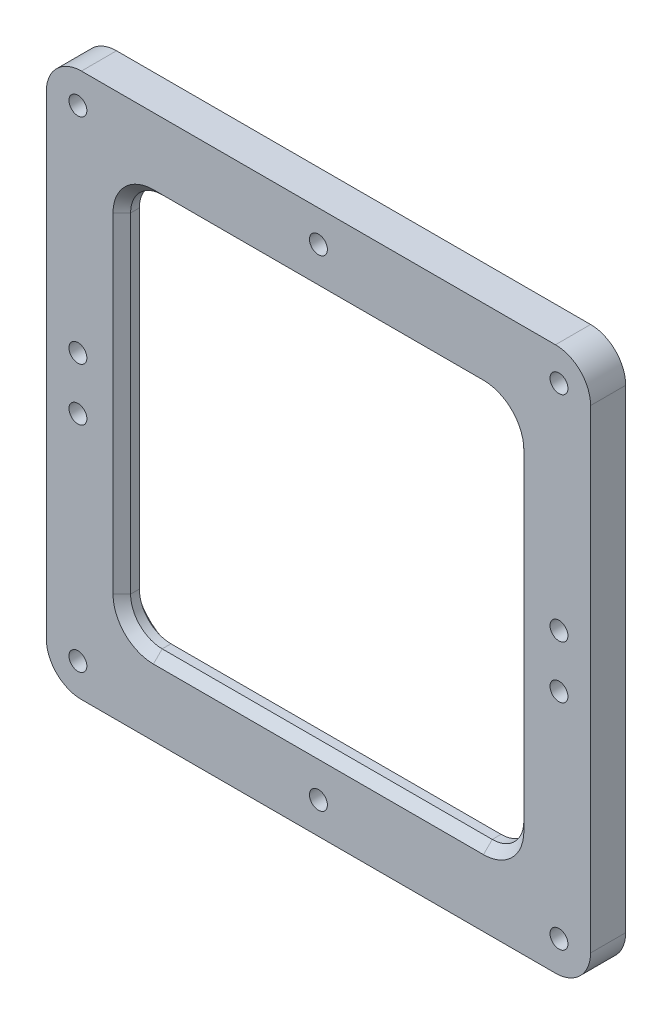
from build123d import *

# Parameters (mm, degrees)
SKETCH_1_W              = 310
SKETCH_1_H              = 310
EXTRUDE_1_DEPTH         = 20
FILLET_1_R              = 20
CUT_EXTRUDE_1_DEPTH     = 10
HOLE_WIZARD_M12_1_D     = 10.2
HOLE_WIZARD_M12_1_DEPTH = 15
HOLE_WIZARD_M12_1_TIP   = 3.064389157
CHAMFER_1_SIZE          = 5


with BuildPart() as part:
    # 草图1 → 凸台-拉伸1 (new body)
    with BuildSketch(Plane.XY):
        Rectangle(SKETCH_1_W, SKETCH_1_H)
        with BuildLine():
            Line((-94, 112), (94, 112))
            ThreePointArc((94, 112), (106.727922061, 106.727922061), (112, 94))
            Line((112, 94), (112, -94))
            ThreePointArc((112, -94), (106.727922061, -106.727922061), (94, -112))
            Line((94, -112), (-94, -112))
            ThreePointArc((-94, -112), (-106.727922061, -106.727922061), (-112, -94))
            Line((-112, -94), (-112, 94))
            ThreePointArc((-112, 94), (-106.727922061, 106.727922061), (-94, 112))
        make_face(mode=Mode.SUBTRACT)
    extrude(amount=EXTRUDE_1_DEPTH)

    # 圆角1
    fillet_1_edges = [part.edges().sort_by_distance(p)[0] for p in [
        (155, -155, 10),
        (-155, -155, 10),
        (-155, 155, 10),
        (155, 155, 10),
    ]]
    fillet(fillet_1_edges, radius=FILLET_1_R)

    # 草图2 → 切除-拉伸1 (cut)
    with BuildSketch(Plane(origin=(0, 0, 0), x_dir=(-1, 0, 0), z_dir=(0, 0, -1))):
        with BuildLine():
            Line((125.1, -95.1), (125.1, 95.1))
            ThreePointArc((125.1, 95.1), (116.313203436, 116.313203436), (95.1, 125.1))
            Line((95.1, 125.1), (-95.1, 125.1))
            ThreePointArc((-95.1, 125.1), (-116.313203436, 116.313203436), (-125.1, 95.1))
            Line((-125.1, 95.1), (-125.1, -95.1))
            ThreePointArc((-125.1, -95.1), (-116.313203436, -116.313203436), (-95.1, -125.1))
            Line((-95.1, -125.1), (95.1, -125.1))
            ThreePointArc((95.1, -125.1), (116.313203436, -116.313203436), (125.1, -95.1))
        make_face()
    extrude(amount=-CUT_EXTRUDE_1_DEPTH, mode=Mode.SUBTRACT)

    # M12 螺纹孔1
    with Locations(Plane(origin=(-137, 137, 20), x_dir=(1, 0, 0), z_dir=(0, 0, 1))):
        with Locations((0, 0), (274, 0), (274, -274), (0, -274), (137, -274), (137, 0), (0, -122), (0, -152), (274, -122), (274, -152)):
            Hole(HOLE_WIZARD_M12_1_D / 2, depth=HOLE_WIZARD_M12_1_DEPTH)
            with Locations((0, 0, -(HOLE_WIZARD_M12_1_DEPTH + HOLE_WIZARD_M12_1_TIP / 2))):  # 118° drill point
                Cone(0, HOLE_WIZARD_M12_1_D / 2, HOLE_WIZARD_M12_1_TIP, mode=Mode.SUBTRACT)

    # 倒角1
    chamfer_1_edges = [part.edges().sort_by_distance(p)[0] for p in [
        (106.727922061, -106.727922061, 20),
        (112, 0, 20),
        (106.727922061, 106.727922061, 20),
        (0, 112, 20),
        (-106.727922061, 106.727922061, 20),
        (-112, 0, 20),
        (-106.727922061, -106.727922061, 20),
        (0, -112, 20),
    ]]
    chamfer(chamfer_1_edges, length=CHAMFER_1_SIZE)


solid = part.part
